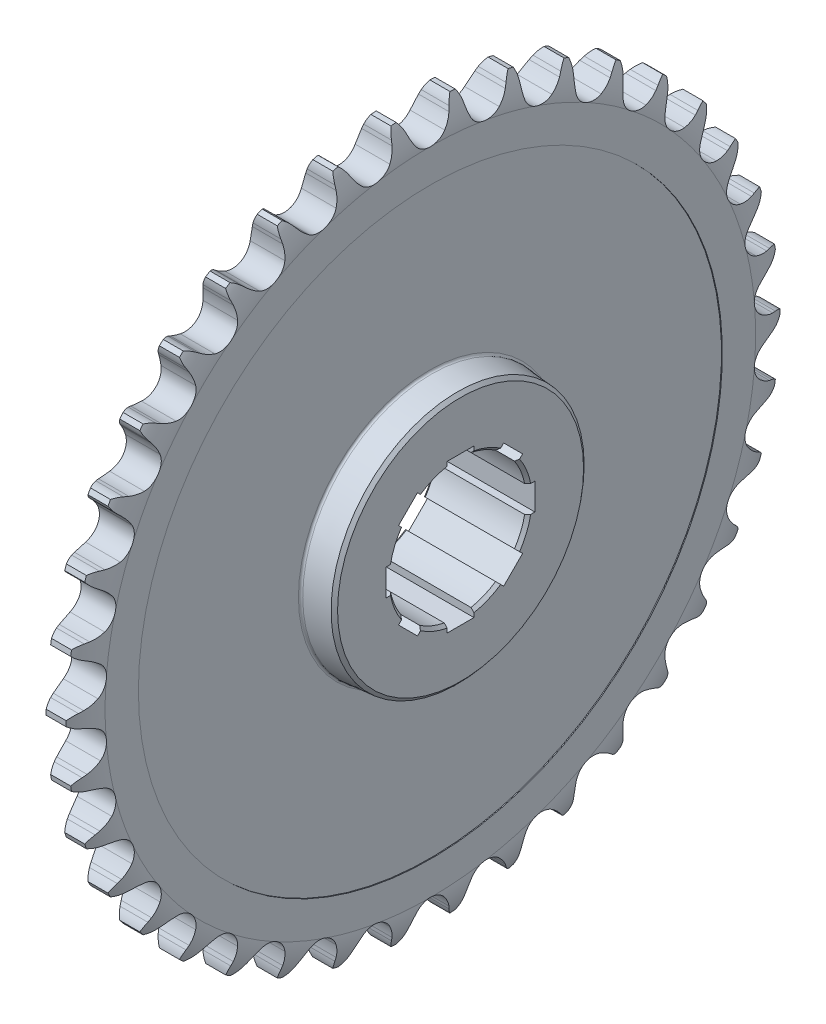
SolidWorks part; units mm, degrees
ref_plane "前视基准面" through (0, 0, 0) normal (0, 0, 1) x (1, 0, 0)
ref_plane "上视基准面" through (0, 0, 0) normal (0, 1, 0) x (1, 0, 0)
ref_plane "右视基准面" through (0, 0, 0) normal (1, 0, 0) x (0, 0, -1)
sketch "草图1" plane through (0, 0, 0) normal (0, 0, 1) x (1, 0, 0)
  line L0 (-9.525, 0) -> (9.525, 0) construction
  line L1 (-5.55, 23) -> (-5.55, 98.1986)
  line L2 (-5.55, 98.1986) -> (-5.8451, 98.1986)
  line L3 (-5.8451, 98.1986) -> (-5.8451, 109.3886)
  line L4 (-3.3686, 120) -> (3.3686, 120)
  line L5 (5.8451, 109.3886) -> (5.8451, 98.1986)
  line L6 (5.8451, 98.1986) -> (5.55, 98.1986)
  line L7 (5.55, 98.1986) -> (5.55, 23)
  line L8 (5.55, 23) -> (-5.55, 23)
  line L9 (0, 0) -> (0, 120) construction
  line L10 (-5.2661, 115.3436) -> (5.2661, 115.3436) construction
  line L11 (-5.2661, -115.3436) -> (5.2661, -115.3436) construction
  line L12 (9.525, 0) -> (47.525, 0) construction
  line L13 (-5.8451, 109.3886) -> (3.7984, 109.3886) construction
  line L14 (-5.8451, -109.3886) -> (3.7984, -109.3886) construction
  line L15 (47.525, 0) -> (59.435, 0) construction
  line L16 (59.435, 0) -> (77.515, 0) construction
  line L17 (77.515, 0) -> (90.085, 0) construction
  line L18 (90.085, 0) -> (112.865, 0) construction
  arc A0 (-3.3686, 120) -> (-5.8451, 109.3886) centre (13.1698, 110.5456) ccw
  arc A1 (3.3686, 120) -> (5.8451, 109.3886) centre (-13.1698, 110.5456) cw
  point P30 (5.8451, 98.1986)
  point P33 (-5.8451, 98.1986)
  dimension "rx" = 19.05
  dimension "d" = 230.6872
  dimension "p" = 19.05
  dimension "z" = 38
  dimension "da" = 240
  dimension "df" = 218.7772
  dimension "dr" = 11.91
  dimension "dk" = 46
  dimension "h" = 18.08
  dimension "bf1" = 11.6901
  dimension "b1" = 12.57
  dimension "ba" = 2.4765
  dimension "pt" = 22.78
  dimension "t" = 11.1
  dimension "C2" = 17.145
revolve "旋转1" add sketch "草图1" angle 360 about L0
sketch "草图2" plane through (0, 0, 0) normal (1, 0, 0) x (0, 0, -1)
  line L0 (0, 0) -> (0, 120) construction
  line L1 (0, 0) -> (-9.9095, 119.5901) construction
  line L2 (0, 0) -> (-19.7514, 118.3634) construction
  line L3 (4.8461, 111.7473) -> (37.4506, 87.5517) construction
  line L4 (6.968, 115.6854) -> (-7.6513, 121.0216) construction
  line L5 (0, 0) -> (9.9095, 119.5901) construction
  line L6 (6.968, 115.6854) -> (7.441, 116.9812)
  line L7 (-6.968, 115.6854) -> (-7.441, 116.9812)
  circle A0 centre (0, 0) radius 120 construction
  arc A1 (4.8461, 111.7473) -> (-4.8461, 111.7473) centre (0, 115.3436) cw
  arc A2 (4.8461, 111.7473) -> (6.968, 115.6854) centre (-7.6513, 121.0216) ccw
  arc A3 (9.025, 119.6601) -> (7.441, 116.9812) centre (15.4301, 114.065) ccw
  arc A4 (-4.8461, 111.7473) -> (-6.968, 115.6854) centre (7.6513, 121.0216) cw
  arc A5 (-9.025, 119.6601) -> (-7.441, 116.9812) centre (-15.4301, 114.065) cw
  arc A7 (9.025, 119.6601) -> (-9.025, 119.6601) centre (0, 0) ccw
  dimension "r1" = 6.0348
  dimension "r3" = 8.5047
  dimension "D1" = 9.474
  dimension "D2" = 4.737
  dimension "α/2" = 53.421
  dimension "M" = 7.6513
  dimension "T" = 5.678
  dimension "β" = 16.526
  dimension "γ/2" = 15.316
  dimension "bc" = 1.3794
extrude "切除-拉伸1" cut sketch "草图2" against normal mid plane 17.5352
pattern_circular "阵列(圆周)1" count 38 over 360 about axis through (0, 0, 0) along (1, 0, 0) of "切除-拉伸1"
sketch "草图4" plane through (-5.55, 0, 0) normal (-1, 0, 0) x (0, 0, 1)
  line L1 (-4.5, 22.5555) -> (4.5, 22.5555)
  line L2 (-4.5, 22.5555) -> (-4.5, 25)
  line L3 (-4.5, 25) -> (4.5, 25)
  line L4 (4.5, 22.5555) -> (4.5, 25)
  circle A0 centre (0, 0) radius 23 construction
  point P6 (0, 25)
  dimension "D1" = 25
  dimension "键槽宽度" = 9
  dimension "t1" = 4.5
sketch "草图5" plane through (0, 0, 0) normal (0, 0, 1) x (1, 0, 0)
  line L1 (-16, 23) -> (16, 23)
  line L2 (-16, 23) -> (-16, 42.4735)
  line L3 (-16, 42.4735) -> (-5.55, 43.3878)
  line L4 (16, 23) -> (16, 42.4735)
  line L6 (0, 0) -> (0, -4.2677) construction
  line L7 (0, 0) -> (-10.4728, 0) construction
  line L8 (-5.55, 23) -> (-5.55, 98.1986) construction
  line L9 (-5.55, 43.3878) -> (5.55, 43.3878)
  line L10 (5.55, 98.1986) -> (5.55, 23) construction
  line L11 (5.55, 43.3878) -> (16, 42.4735)
  dimension "D1" = 5
  dimension "L" = 32
  dimension "H" = 19.4735
revolve "旋转2" add sketch "草图5" angle 360 about L7
extrude "切除-拉伸2" cut sketch "草图4" against normal through all
mirror "镜向1" about plane through (0, 0, 0) normal (1, 0, 0) of "切除-拉伸2"
fillet "圆角1" radius 0.762 2 edges at (5.55, 0, -43.3878) (-5.55, 0, -43.3878)
chamfer "倒角1" distance 1 angle 45 4 edges at (16, -23, 0) (16, 0, -42.4735) (-16, -23, 0) (-16, 0, -42.4735)
sketch "草图6" plane through (-5.55, 0, 0) normal (-1, 0, 0) x (0, 0, 1)
  line L0 (0, 98.1986) -> (0, 75.9986) construction
  line L1 (0, 75.9986) -> (0, 66.286) construction
  line L2 (0, 66.286) -> (0, 44.086) construction
  line L3 (0, 44.086) -> (0, 0) construction
  circle A0 centre (0, 71.1423) radius 4.8563
  circle A1 centre (0, 0) radius 98.1986 construction
  circle A2 centre (0, 0) radius 98.1986 construction
  circle A3 centre (0, 0) radius 44.086 construction
  dimension "g" = 22.2
pattern_circular "阵列(圆周)3" count 8 over 360 of "切除-拉伸2", "镜向1"
